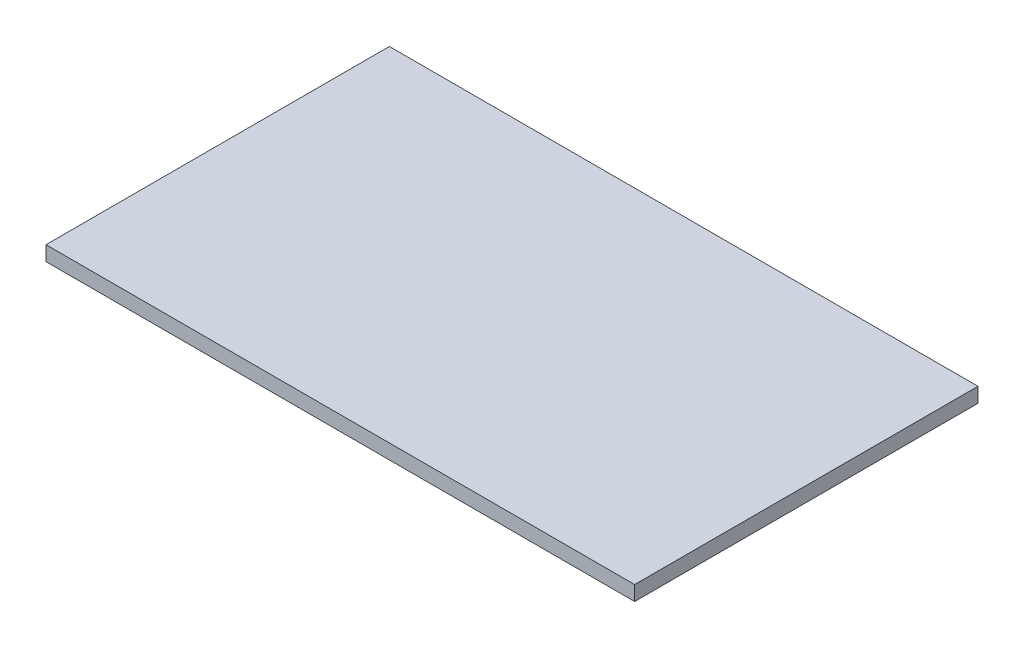
SolidWorks part; units mm, degrees
ref_plane "前视基准面" through (0, 0, 0) normal (0, 0, 1) x (1, 0, 0)
ref_plane "上视基准面" through (0, 0, 0) normal (0, 1, 0) x (1, 0, 0)
ref_plane "右视基准面" through (0, 0, 0) normal (1, 0, 0) x (0, 0, -1)
sketch "草图1" plane through (0, 0, 0) normal (0, 0, 1) x (1, 0, 0)
  line L1 (60, -1.5) -> (-60, -1.5)
  line L2 (60, -1.5) -> (60, 1.5)
  line L3 (60, 1.5) -> (-60, 1.5)
  line L4 (-60, -1.5) -> (-60, 1.5)
  line L5 (60, -1.5) -> (-60, 1.5) construction
  line L6 (60, 1.5) -> (-60, -1.5) construction
  point P0 (0, 0)
  dimension "D1" = 3
  dimension "D2" = 120
extrude "凸台-拉伸1" add sketch "草图1" along normal blind 70
sketch "草图2" plane through (0, -1.5, 0) normal (0, -1, 0) x (1, 0, 0)
  line L0 (-60, 70) -> (-60, 0) construction
  line L1 (-30, 31) -> (-60, 31)
  line L2 (-30, 31) -> (-30, 39)
  line L3 (-30, 39) -> (-60, 39)
  line L4 (-60, 31) -> (-60, 39)
  line L5 (-30, 31) -> (-60, 39) construction
  line L6 (-30, 39) -> (-60, 31) construction
  line L7 (60, 35) -> (-30, 35) construction
  line L8 (60, 70) -> (60, 0) construction
  point P0 (-45, 35)
  dimension "D1" = 8
  dimension "D2" = 30
